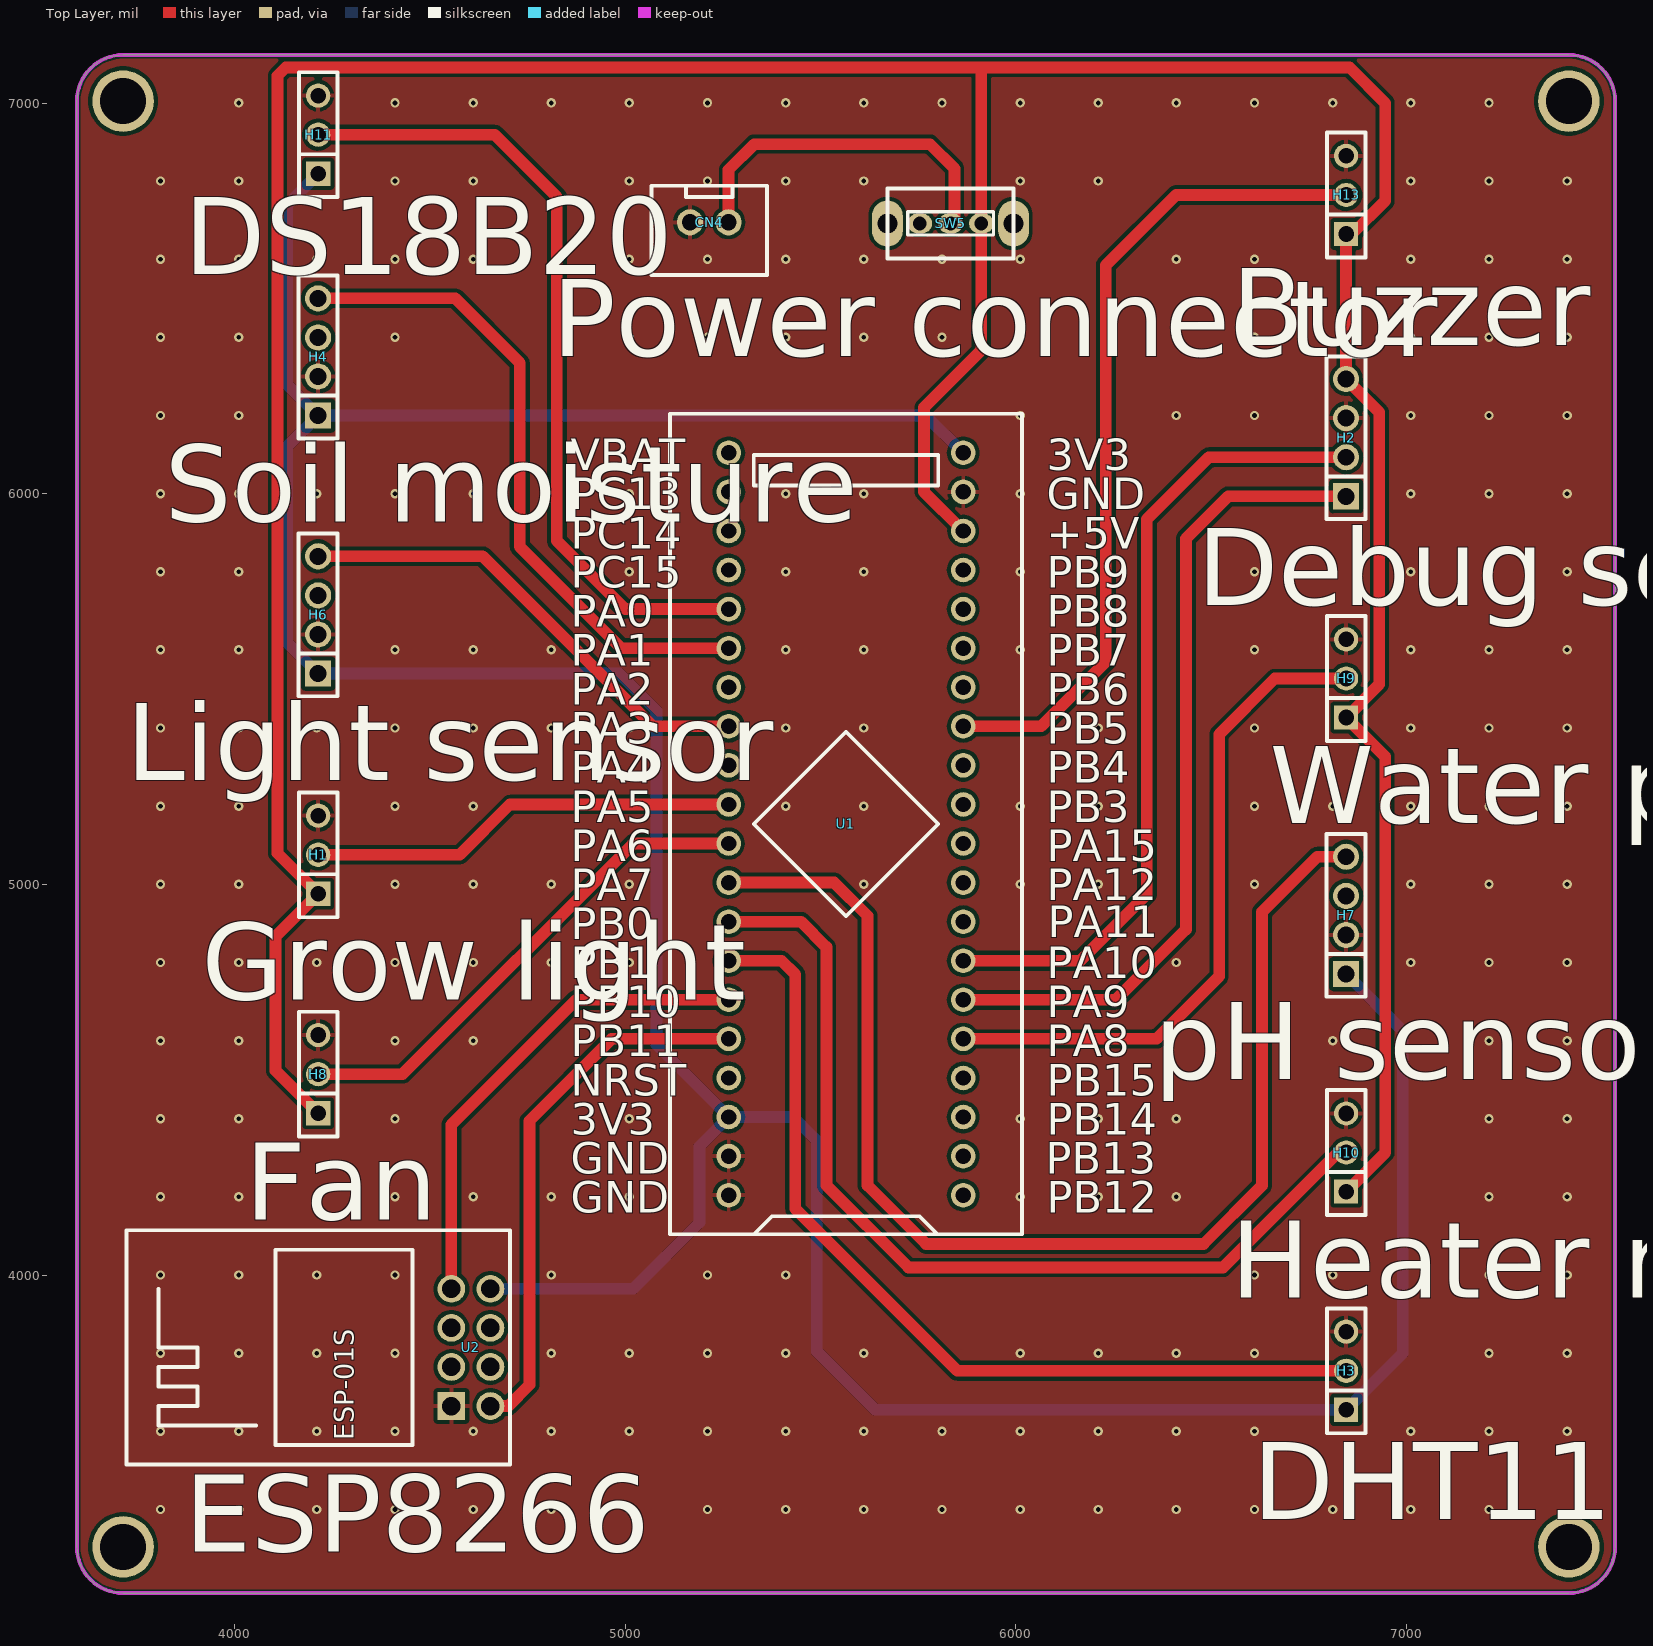
[diagram p0: Top Layer view]
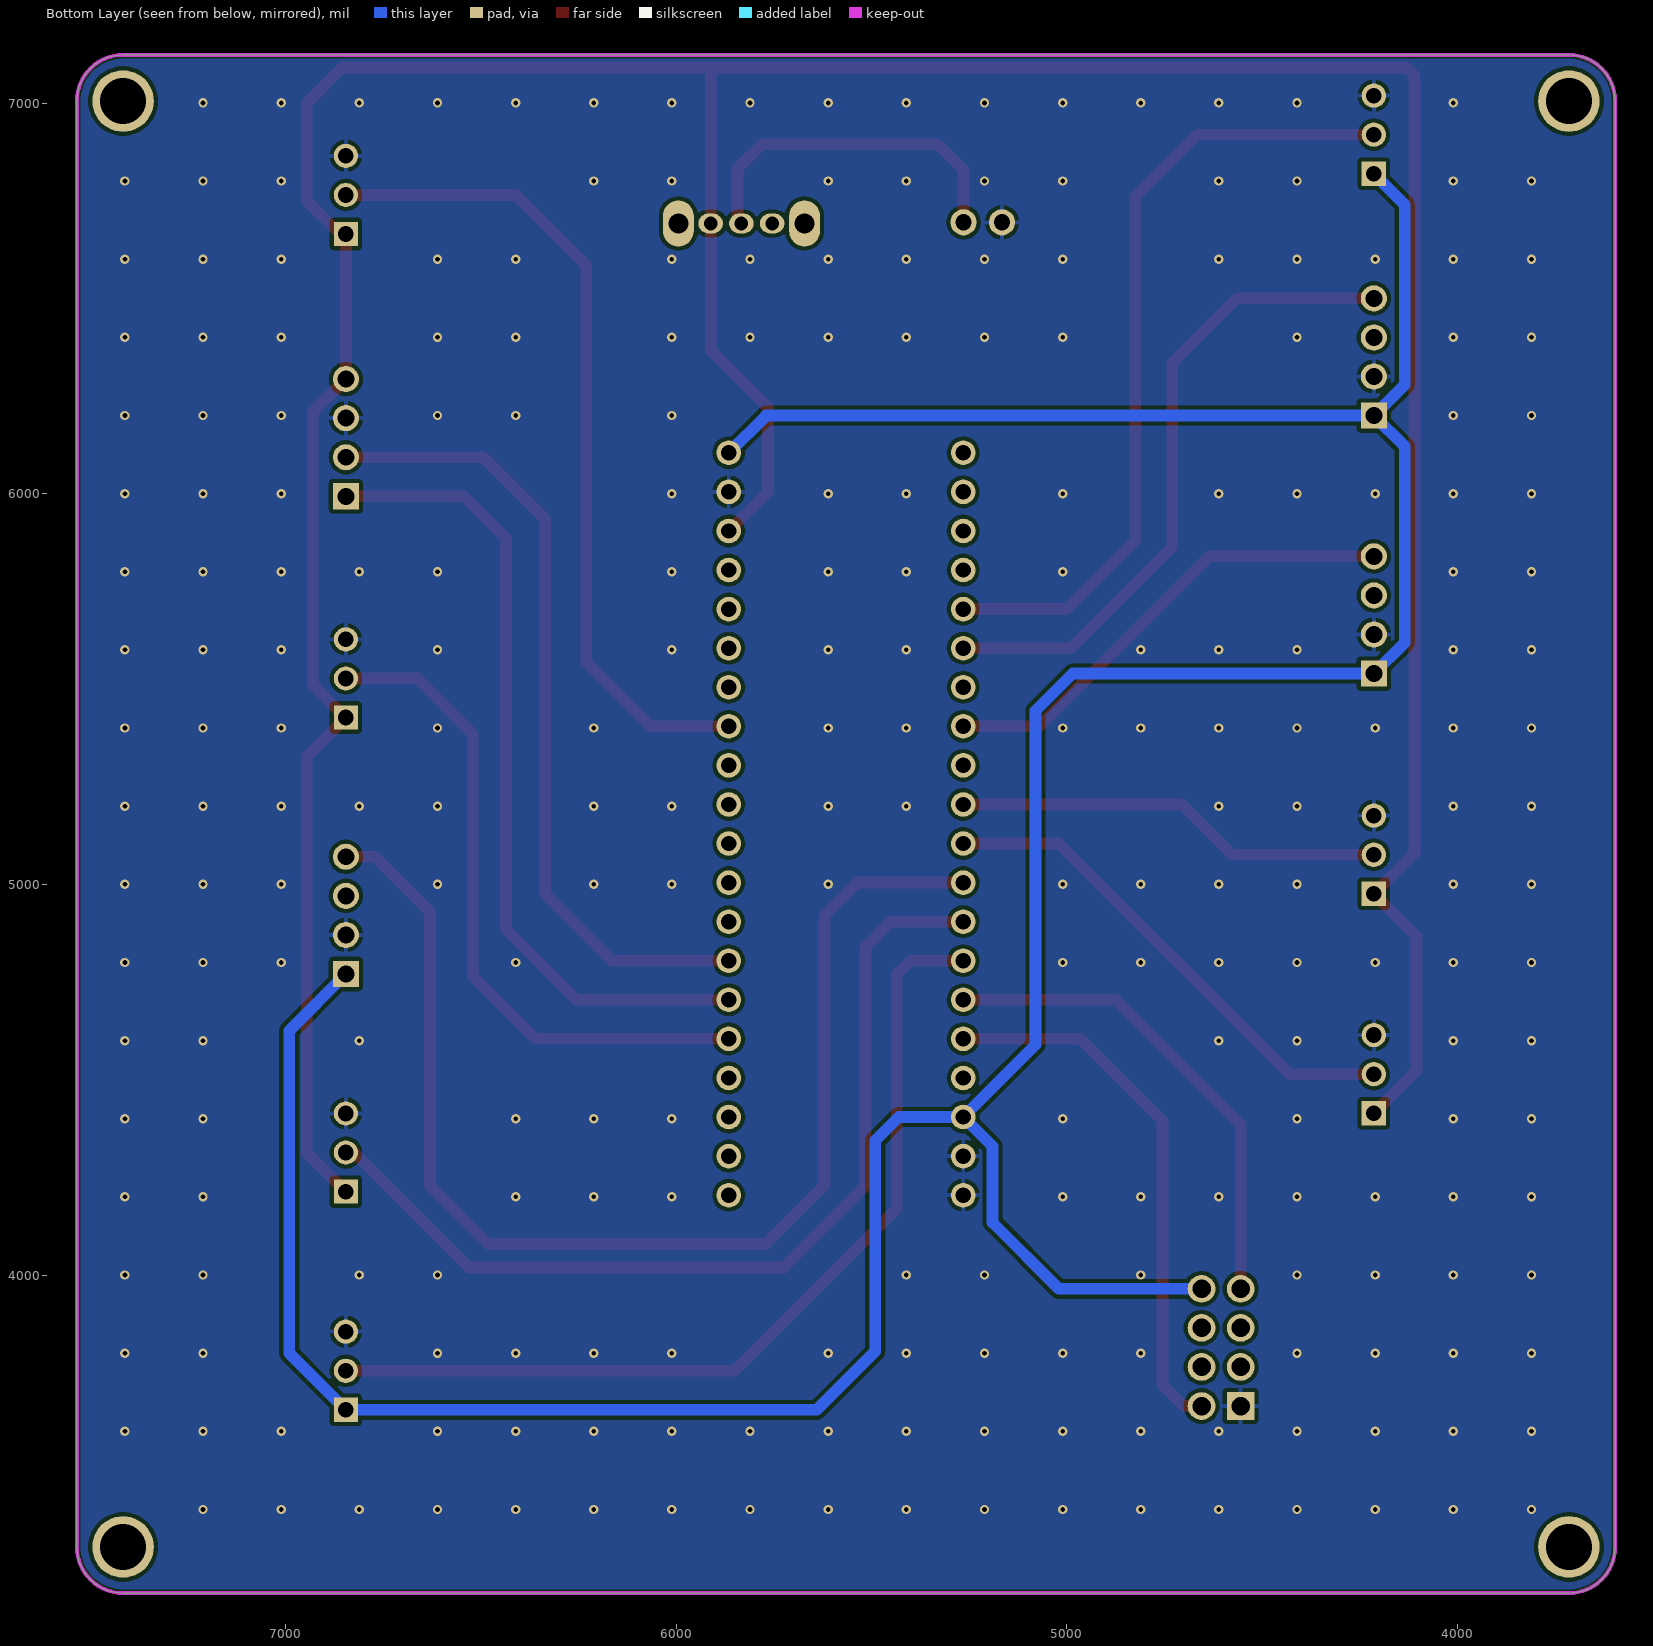
[diagram p1: Bottom Layer view, seen from below]
# Altium PCB MISC89003.pcbdoc
Units mil, origin at the board's own origin, x right, y up, seen from the top; angles counter-clockwise.
Board outline 3937.01 x 3937.01 mil, 2 copper layers (Top Layer, Bottom Layer), stack 62.206 mil thick; 15 components, 38 nets, 96 pads, 243 vias.

## Layer stack, top to bottom
Top Solder Mask Layer: solder mask 0.394, Dk 3.3
Top Layer: signal copper 1.379
Dielectric1: surface 59.449, FR4, Dk 4.5
Bottom Layer: signal copper 1.378
Bottom Solder Mask Layer: solder mask 0.394, Dk 3.3

## Board outline
3714.61,7123.5 ccw(c3714.61,7005.39) 3596.5,7005.39 3596.5,3304.61 ccw(c3714.61,3304.61) 3714.61,3186.5 7415.39,3186.5 ccw(c7415.39,3304.61) 7533.5,3304.61 7533.5,7005.39 ccw(c7415.39,7005.39) 7415.39,7123.5 3714.61,7123.5

## Design rules (kind name [scope] priority, off if disabled: settings)
BoardOutlineClearance copperThickness2oz_1 [All] p2 off: genericclearance=7.99 ignorepadtopadclearanceinfootprint=FALSE except(0: Arc-SplitContinuation Track-SplitContinuation SMDPad-SplitContinuation THPad-SplitContinuation Via-SplitContinuation Fill-SplitContinuation Region-SplitContinuation Poly-SplitContinuation Text-SplitContinuation Hole-SplitContinuation; 5.98: Arc-CutoutEdge Track-CutoutEdge SMDPad-CutoutEdge THPad-CutoutEdge Via-CutoutEdge Text-CutoutEdge; 6.9: Hole-OutlineEdge Hole-CutoutEdge; 10: Poly-OutlineEdge Poly-CutoutEdge; 11.81: Arc-OutlineEdge Track-OutlineEdge SMDPad-OutlineEdge THPad-OutlineEdge Via-OutlineEdge Fill-OutlineEdge Region-OutlineEdge Text-OutlineEdge Fill-CutoutEdge Region-CutoutEdge)
BoardOutlineClearance Plane_innerPlane_1 [All] p4 off: genericclearance=4.02 ignorepadtopadclearanceinfootprint=FALSE except(0: Arc-SplitContinuation Track-SplitContinuation SMDPad-SplitContinuation THPad-SplitContinuation Via-SplitContinuation Fill-SplitContinuation Region-SplitContinuation Poly-SplitContinuation Text-SplitContinuation Hole-SplitContinuation; 5.98: Arc-CutoutEdge Track-CutoutEdge SMDPad-CutoutEdge THPad-CutoutEdge Via-CutoutEdge Text-CutoutEdge; 6.9: Hole-OutlineEdge Hole-CutoutEdge; 10: Poly-OutlineEdge Poly-CutoutEdge; 11.81: Arc-OutlineEdge Track-OutlineEdge SMDPad-OutlineEdge THPad-OutlineEdge Via-OutlineEdge Fill-OutlineEdge Region-OutlineEdge Text-OutlineEdge Fill-CutoutEdge Region-CutoutEdge)
BoardOutlineClearance Copper_copperRegion_1 [All] p6 off: genericclearance=4.02 ignorepadtopadclearanceinfootprint=FALSE except(0: Arc-SplitContinuation Track-SplitContinuation SMDPad-SplitContinuation THPad-SplitContinuation Via-SplitContinuation Fill-SplitContinuation Region-SplitContinuation Poly-SplitContinuation Text-SplitContinuation Hole-SplitContinuation; 5.98: Arc-CutoutEdge Track-CutoutEdge SMDPad-CutoutEdge THPad-CutoutEdge Via-CutoutEdge Text-CutoutEdge; 6.9: Hole-OutlineEdge Hole-CutoutEdge; 10: Poly-OutlineEdge Poly-CutoutEdge; 11.81: Arc-OutlineEdge Track-OutlineEdge SMDPad-OutlineEdge THPad-OutlineEdge Via-OutlineEdge Fill-OutlineEdge Region-OutlineEdge Text-OutlineEdge Fill-CutoutEdge Region-CutoutEdge)
BoardOutlineClearance Copper_copperRegion_copperThickness1oz_1 [All] p8 off: genericclearance=4.02 ignorepadtopadclearanceinfootprint=FALSE except(0: Arc-SplitContinuation Track-SplitContinuation SMDPad-SplitContinuation THPad-SplitContinuation Via-SplitContinuation Fill-SplitContinuation Region-SplitContinuation Poly-SplitContinuation Text-SplitContinuation Hole-SplitContinuation; 5.98: Arc-CutoutEdge Track-CutoutEdge SMDPad-CutoutEdge THPad-CutoutEdge Via-CutoutEdge Text-CutoutEdge; 6.9: Hole-OutlineEdge Hole-CutoutEdge; 10: Poly-OutlineEdge Poly-CutoutEdge; 11.81: Arc-OutlineEdge Track-OutlineEdge SMDPad-OutlineEdge THPad-OutlineEdge Via-OutlineEdge Fill-OutlineEdge Region-OutlineEdge Text-OutlineEdge Fill-CutoutEdge Region-CutoutEdge)
BoardOutlineClearance Copper_copperRegion_Copper_copperRegion_1 [All] p10 off: genericclearance=4.02 ignorepadtopadclearanceinfootprint=FALSE except(0: Arc-SplitContinuation Track-SplitContinuation SMDPad-SplitContinuation THPad-SplitContinuation Via-SplitContinuation Fill-SplitContinuation Region-SplitContinuation Poly-SplitContinuation Text-SplitContinuation Hole-SplitContinuation; 5.98: Arc-CutoutEdge Track-CutoutEdge SMDPad-CutoutEdge THPad-CutoutEdge Via-CutoutEdge Text-CutoutEdge; 6.9: Hole-OutlineEdge Hole-CutoutEdge; 10: Poly-OutlineEdge Poly-CutoutEdge; 11.81: Arc-OutlineEdge Track-OutlineEdge SMDPad-OutlineEdge THPad-OutlineEdge Via-OutlineEdge Fill-OutlineEdge Region-OutlineEdge Text-OutlineEdge Fill-CutoutEdge Region-CutoutEdge)
BoardOutlineClearance copperThickness1oz_1 [All] p12: genericclearance=4.02 ignorepadtopadclearanceinfootprint=FALSE except(0: Arc-SplitContinuation Track-SplitContinuation SMDPad-SplitContinuation THPad-SplitContinuation Via-SplitContinuation Fill-SplitContinuation Region-SplitContinuation Poly-SplitContinuation Text-SplitContinuation Hole-SplitContinuation; 5.98: Arc-CutoutEdge Track-CutoutEdge SMDPad-CutoutEdge THPad-CutoutEdge Via-CutoutEdge Text-CutoutEdge; 6.9: Hole-OutlineEdge Hole-CutoutEdge; 10: Poly-OutlineEdge Poly-CutoutEdge; 11.81: Arc-OutlineEdge Track-OutlineEdge SMDPad-OutlineEdge THPad-OutlineEdge Via-OutlineEdge Fill-OutlineEdge Region-OutlineEdge Text-OutlineEdge Fill-CutoutEdge Region-CutoutEdge)
Clearance copperThickness2oz [All] p1 off: gap=7.99 ignorepadtopadclearanceinfootprint=FALSE except(5.98: SMDPad-Track SMDPad-SMDPad THPad-Track SMDPad-THPad THPad-THPad Track-Via SMDPad-Via THPad-Via Via-Via Fill-SMDPad Region-SMDPad Fill-THPad Region-THPad Fill-Via Region-Via Fill-Fill Fill-Region Region-Region Arc-Track Arc-SMDPad Arc-THPad Arc-Via Fill-Arc Region-Arc Arc-Arc Text-Track SMDPad-Text Text-THPad Text-Via Fill-Text Region-Text Arc-Text Text-Text; 6.9: Hole-Track Hole-SMDPad Hole-THPad Hole-Via Fill-Hole Region-Hole Hole-Arc Hole-Text; 10: Poly-Track Poly-SMDPad Poly-THPad Poly-Via Poly-Fill Poly-Region Poly-Poly Poly-Arc Poly-Text Poly-Hole; 11.81: Fill-Track Region-Track)
Clearance Plane_innerPlane [All] p3 off: gap=4.02 ignorepadtopadclearanceinfootprint=FALSE except(5.98: SMDPad-Track SMDPad-SMDPad THPad-Track SMDPad-THPad THPad-THPad Track-Via SMDPad-Via THPad-Via Via-Via Fill-SMDPad Region-SMDPad Fill-THPad Region-THPad Fill-Via Region-Via Fill-Fill Fill-Region Region-Region Arc-Track Arc-SMDPad Arc-THPad Arc-Via Fill-Arc Region-Arc Arc-Arc Text-Track SMDPad-Text Text-THPad Text-Via Fill-Text Region-Text Arc-Text Text-Text; 6.9: Hole-Track Hole-SMDPad Hole-THPad Hole-Via Fill-Hole Region-Hole Hole-Arc Hole-Text; 10: Poly-Track Poly-SMDPad Poly-THPad Poly-Via Poly-Fill Poly-Region Poly-Poly Poly-Arc Poly-Text Poly-Hole; 11.81: Fill-Track Region-Track)
Clearance Copper_copperRegion [All] p5 off: gap=4.02 ignorepadtopadclearanceinfootprint=FALSE except(5.98: SMDPad-Track SMDPad-SMDPad THPad-Track SMDPad-THPad THPad-THPad Track-Via SMDPad-Via THPad-Via Via-Via Fill-SMDPad Region-SMDPad Fill-THPad Region-THPad Fill-Via Region-Via Fill-Fill Fill-Region Region-Region Arc-Track Arc-SMDPad Arc-THPad Arc-Via Fill-Arc Region-Arc Arc-Arc Text-Track SMDPad-Text Text-THPad Text-Via Fill-Text Region-Text Arc-Text Text-Text; 6.9: Hole-Track Hole-SMDPad Hole-THPad Hole-Via Fill-Hole Region-Hole Hole-Arc Hole-Text; 10: Poly-Track Poly-SMDPad Poly-THPad Poly-Via Poly-Fill Poly-Region Poly-Poly Poly-Arc Poly-Text Poly-Hole; 11.81: Fill-Track Region-Track)
Clearance Copper_copperRegion_copperThickness1oz [All] p7 off: gap=4.02 ignorepadtopadclearanceinfootprint=FALSE except(5.98: SMDPad-Track SMDPad-SMDPad THPad-Track SMDPad-THPad THPad-THPad Track-Via SMDPad-Via THPad-Via Via-Via Fill-SMDPad Region-SMDPad Fill-THPad Region-THPad Fill-Via Region-Via Fill-Fill Fill-Region Region-Region Arc-Track Arc-SMDPad Arc-THPad Arc-Via Fill-Arc Region-Arc Arc-Arc Text-Track SMDPad-Text Text-THPad Text-Via Fill-Text Region-Text Arc-Text Text-Text; 6.9: Hole-Track Hole-SMDPad Hole-THPad Hole-Via Fill-Hole Region-Hole Hole-Arc Hole-Text; 10: Poly-Track Poly-SMDPad Poly-THPad Poly-Via Poly-Fill Poly-Region Poly-Poly Poly-Arc Poly-Text Poly-Hole; 11.81: Fill-Track Region-Track)
Clearance Copper_copperRegion_Copper_copperRegion [All] p9 off: gap=4.02 ignorepadtopadclearanceinfootprint=FALSE except(5.98: SMDPad-Track SMDPad-SMDPad THPad-Track SMDPad-THPad THPad-THPad Track-Via SMDPad-Via THPad-Via Via-Via Fill-SMDPad Region-SMDPad Fill-THPad Region-THPad Fill-Via Region-Via Fill-Fill Fill-Region Region-Region Arc-Track Arc-SMDPad Arc-THPad Arc-Via Fill-Arc Region-Arc Arc-Arc Text-Track SMDPad-Text Text-THPad Text-Via Fill-Text Region-Text Arc-Text Text-Text; 6.9: Hole-Track Hole-SMDPad Hole-THPad Hole-Via Fill-Hole Region-Hole Hole-Arc Hole-Text; 10: Poly-Track Poly-SMDPad Poly-THPad Poly-Via Poly-Fill Poly-Region Poly-Poly Poly-Arc Poly-Text Poly-Hole; 11.81: Fill-Track Region-Track)
Clearance copperThickness1oz [All] p11: gap=4.02 ignorepadtopadclearanceinfootprint=FALSE except(5.98: SMDPad-Track SMDPad-SMDPad THPad-Track SMDPad-THPad THPad-THPad Track-Via SMDPad-Via THPad-Via Via-Via Fill-SMDPad Region-SMDPad Fill-THPad Region-THPad Fill-Via Region-Via Fill-Fill Fill-Region Region-Region Arc-Track Arc-SMDPad Arc-THPad Arc-Via Fill-Arc Region-Arc Arc-Arc Text-Track SMDPad-Text Text-THPad Text-Via Fill-Text Region-Text Arc-Text Text-Text; 6.9: Hole-Track Hole-SMDPad Hole-THPad Hole-Via Fill-Hole Region-Hole Hole-Arc Hole-Text; 10: Poly-Track Poly-SMDPad Poly-THPad Poly-Via Poly-Fill Poly-Region Poly-Poly Poly-Arc Poly-Text Poly-Hole; 11.81: Fill-Track Region-Track)
DiffPairsRouting differentialPair [All] p1: maxlimit=6 minlimit=6 mostfreqgap=6 toplayer_minwidth=5 toplayer_prefwidth=10 toplayer_maxwidth=100 toplayer_mingap=6 toplayer_prefgap=6 toplayer_maxgap=6 bottomlayer_minwidth=5 bottomlayer_prefwidth=10 bottomlayer_maxwidth=100 bottomlayer_mingap=6 bottomlayer_prefgap=6 bottomlayer_maxgap=6 maxuncoupledlength=10
HoleToHoleClearance otherClearance [All] p1: gap=11.81 allowstackedmicrovias=TRUE
Length netLength [All] p1: minlimit=0 maxlimit=0
PasteMaskExpansion pasteMaskExpansion [All] p1: expansion=0
PlaneConnect innerPlane [All] p1: planeconnectstyle=Relief reliefexpansion=20 reliefentries=4 reliefconductorwidth=10 reliefairgap=10
PolygonConnect copperRegion_copperThickness1oz [All] p1 off: connectstyle=Relief reliefconductorwidth=10 reliefentries=4 polygonreliefangle="90 Angle" airgapwidth=10 via.connectstyle=Relief via.reliefconductorwidth=10 via.reliefentries=4 via.polygonreliefangle="90 Angle" via.airgapwidth=10
PolygonConnect copperRegion_Copper_copperRegion [All] p2 off: connectstyle=Relief reliefconductorwidth=10 reliefentries=4 polygonreliefangle="90 Angle" airgapwidth=10 via.connectstyle=Relief via.reliefconductorwidth=10 via.reliefentries=4 via.polygonreliefangle="90 Angle" via.airgapwidth=10
PolygonConnect copperRegion [All] p3: connectstyle=Relief reliefconductorwidth=10 reliefentries=4 polygonreliefangle="90 Angle" airgapwidth=10 via.connectstyle=Relief via.reliefconductorwidth=10 via.reliefentries=4 via.polygonreliefangle="90 Angle" via.airgapwidth=10
RoutingVias viaSize [All] p1: holewidth=12.01 width=24.02 viastyle="Through Hole" minholewidth=11.81 minwidth=19.68 maxholewidth=248.03 maxwidth=393.7
SolderMaskExpansion solderMaskExpansion [IsVia] p1: expansion=-1000 istentingtop=TRUE
SolderMaskExpansion solderMaskExpansion [All] p2: expansion=2 istentingtop=FALSE
Width copperThickness2oz_2 [All] p1 off: maxlimit=100 minlimit=8 preferedwidth=10
Width copperThickness1oz_2 [All] p2: maxlimit=100 minlimit=5 preferedwidth=10

## Components (designator, comment, footprint, x,y, rotation, side; value= is the part's Value field where it differs from the comment)
CN4 "XH2.54*2P_straight" CONN-TH_2P-P2.50-XH2.54-2P 5215,6695 r0 top
H1 "" HDR-TH_3P-P2.54-V-F 4214,5076.28 r90 top
H2 "" HDR-TH_4P-P2.54-V-F 6845,6143.71 r90 top
H3 "" HDR-TH_3P-P2.54-V-F 6845,3755.57 r90 top
H4 "" HDR-TH_4P-P2.54-V-F 4214,6350.33 r90 top
H6 "" HDR-TH_4P-P2.54-V-F 4214,5690.14 r90 top
H7 "" HDR-TH_4P-P2.54-V-F 6845,4921.1 r90 top
H8 "" HDR-TH_3P-P2.54-V-F 4214,4514.73 r90 top
H9 "" HDR-TH_3P-P2.54-V-F 6845,5527.48 r90 top
H10 "" HDR-TH_3P-P2.54-V-F 6845,4314.12 r90 top
H11 "" HDR-TH_3P-P2.54-V-F 4214,6919.25 r90 top
H13 "" HDR-TH_3P-P2.54-V-F 6845,6765 r90 top
SW5 "" 拨动开关 5837.9,6692.05 r180 top
U1 "STM32F103C8T6-Card" CONN-TH_L53.3-W22.9_STM32F103C8T6-CARD 5565,5155 r90 top
U2 "ESP-01S" WIFIM-TH_ESP-01S 4605,3815.3 r90 top

## Footprints (in the part's own frame and the unit in brackets; to place one, negate y for a bottom-side part, rotate by r counter-clockwise, add the part's x,y. Pads: shape width x height; smd on the part's side, far side on the other; paste and mask are expansions set on the pad)
CONN-TH_2P-P2.50-XH2.54-2P [mm]
  round 1.7 hole 1.05 paste+0 mask+0.05: 1(1.25,0) 2(-1.25,0)
  silkscreen extent -3.75,-3.42 3.75,2.37
CONN-TH_L53.3-W22.9_STM32F103C8T6-CARD [mm]
  round 1.6 hole 1: 1(-24.13,-7.62) 2(-21.59,-7.62) 3(-19.05,-7.62) 4(-16.51,-7.62) 5(-13.97,-7.62) 6(-11.43,-7.62) 7(-8.89,-7.62) 8(-6.35,-7.62) 9(-3.81,-7.62) 10(-1.27,-7.62) 11(1.27,-7.62) 12(3.81,-7.62) 13(6.35,-7.62) 14(8.89,-7.62) 15(11.43,-7.62) 16(13.97,-7.62) 17(16.51,-7.62) 18(19.05,-7.62) 19(21.59,-7.62) 20(24.13,-7.62) 21(24.13,7.62) 22(21.59,7.62) 23(19.05,7.62) 24(16.51,7.62) 25(13.97,7.62) 26(11.43,7.62) 27(8.89,7.62) 28(6.35,7.62) 29(3.81,7.62) 30(1.27,7.62) 31(-1.27,7.62) 32(-3.81,7.62) 33(-6.35,7.62) 34(-8.89,7.62) 35(-11.43,7.62) 36(-13.97,7.62) 37(-16.51,7.62) 38(-19.05,7.62) 39(-21.59,7.62) 40(-24.13,7.62)
  silkscreen extent -26.67,-11.43 26.67,11.43
HDR-TH_3P-P2.54-V-F [mil]
  rect 62x62 hole 40.16: 1(-100,0)
  round 62 hole 40.16: 2(0,0) 3(100,0)
  silkscreen extent -160,-49 160,49
HDR-TH_4P-P2.54-V-F [mm]
  rect 1.7x1.7 hole 1.1: 1(-3.81,0)
  round 1.7 hole 1.1: 2(-1.27,0) 3(1.27,0) 4(3.81,0)
  silkscreen extent -5.29,-1.27 5.29,1.27
WIFIM-TH_ESP-01S [mm]
  rect 1.8x1.8 hole 1.2: 1(-3.81,1.27)
  round 1.8 hole 1.2: 2(-1.27,1.27) 3(1.27,1.27) 4(3.81,1.27) 5(3.81,-1.27) 6(1.27,-1.27) 7(-1.27,-1.27) 8(-3.81,-1.27)
  silkscreen extent -7.62,-2.54 7.62,22.4
拨动开关 [mil]
  oval 63x51.2 hole 35.4 paste+0 mask+2: 1(-73.4,0) 2(5,0) 3(84,0)
  oval 78.7x118.1 hole 51.2 paste+0 mask+2: 4(166.7,0) 5(-156.1,0)
  silkscreen extent -156,-90 167,90

## Free pads (board coordinates)
  round 157.48 hole 118.11: 1(3714.61,7005.39) 1(3714.61,3304.61) 1(7415.39,7005.39) 1(7415.39,3304.61)

## Via types
v1: diameter 24.02, hole 12, Top Layer to Bottom Layer, 243 vias

## Nets (pads, with @x,y where several pads share a name; then routed paths per layer and width w, separated by ;. In a path a pad name is that pad's centre, name@x,y a point inside that pad or via, vN(x,y) a via of type N, cw(c..) or ccw(c..) an arc to the next point about the centre after c; other vN are vias at no path point)
$1N17118: CN4.1 SW5.2 | length 906.3
  Top Layer w30: CN4.1 5264.22,6829.22 5330,6895 5780,6895 5842.9,6832.1 SW5.2@5842.9,6692.05
+5V: H1.1 H2.4 H8.1 H9.1 H10.1 H13.1 SW5.1 U1.18 | length 9949
  Top Layer w30: H8.1 4105,4523.73 4105,4867.28 H1.1 4110,5080.28 4110,7070 4131.21,7091.21 5909.46,7091.21 ; U1.18 5764.5,6005.5 5764.5,6220.75 5911.3,6367.55 SW5.1 5911.3,7089.37 5909.46,7091.21 ; H10.1 6945,4314.12 6945,5327.48 H9.1 6930,5512.48 6930,6208.71 H2.4 H13.1 6860,6665 6945,6750 6945,7000 6853.79,7091.21 5909.46,7091.21
GND: CN4.2 H1.3 H2.3 H3.3 H4.2 H6.2 H7.2 H8.3 H9.3 H10.3 H11.3 H13.3 U1.19 U1.39 U1.40 U2.1
  other v1: 3810.6,3400.6 4010.6,3400.6 4210.6,3400.6 4410.6,3400.6 4610.6,3400.6 4810.6,3400.6 5010.6,3400.6 5210.6,3400.6 5410.6,3400.6 5610.6,3400.6 5810.6,3400.6 6010.6,3400.6 6210.6,3400.6 6410.6,3400.6 6610.6,3400.6 6810.6,3400.6 7010.6,3400.6 7210.6,3400.6 3810.6,3600.6 4010.6,3600.6 4210.6,3600.6 4410.6,3600.6 4610.6,3600.6 4810.6,3600.6 5010.6,3600.6 5210.6,3600.6 5410.6,3600.6 5610.6,3600.6 5810.6,3600.6 6010.6,3600.6 6210.6,3600.6 6410.6,3600.6 6610.6,3600.6 7010.6,3600.6 7210.6,3600.6 7410.6,3600.6 3810.6,3800.6 4010.6,3800.6 4210.6,3800.6 4410.6,3800.6 4810.6,3800.6 5010.6,3800.6 5210.6,3800.6 5410.6,3800.6 5610.6,3800.6 6010.6,3800.6 6210.6,3800.6 6410.6,3800.6 6610.6,3800.6 7210.6,3800.6 7410.6,3800.6 3810.6,4000.6 4010.6,4000.6 4210.6,4000.6 4410.6,4000.6 4810.6,4000.6 5210.6,4000.6 5410.6,4000.6 6610.6,4000.6 6810.6,4000.6 7210.6,4000.6 7410.6,4000.6 3810.6,4200.6 4010.6,4200.6 4210.6,4200.6 4410.6,4200.6 4610.6,4200.6 4810.6,4200.6 5010.6,4200.6 6010.6,4200.6 6210.6,4200.6 6410.6,4200.6 7210.6,4200.6 7410.6,4200.6 3810.6,4400.6 4010.6,4400.6 4410.6,4400.6 5010.6,4400.6 6010.6,4400.6 6210.6,4400.6 6410.6,4400.6 7210.6,4400.6 7410.6,4400.6 3810.6,4600.6 4010.6,4600.6 4410.6,4600.6 4610.6,4600.6 6810.6,4600.6 7210.6,4600.6 7410.6,4600.6 3810.6,4800.6 4010.6,4800.6 4210.6,4800.6 4410.6,4800.6 4610.6,4800.6 4810.6,4800.6 5010.6,4800.6 6410.6,4800.6 7010.6,4800.6 7210.6,4800.6 7410.6,4800.6 3810.6,5000.6 4010.6,5000.6 4410.6,5000.6 4610.6,5000.6 4810.6,5000.6 5010.6,5000.6 5610.6,5000.6 6010.6,5000.6 6210.6,5000.6 6610.6,5000.6 7010.6,5000.6 7210.6,5000.6 7410.6,5000.6 3810.6,5200.6 4010.6,5200.6 4410.6,5200.6 4610.6,5200.6 5410.6,5200.6 5610.6,5200.6 6010.6,5200.6 6210.6,5200.6 6610.6,5200.6 6810.6,5200.6 7010.6,5200.6 7210.6,5200.6 7410.6,5200.6 3810.6,5400.6 4010.6,5400.6 4210.6,5400.6 4410.6,5400.6 4610.6,5400.6 4810.6,5400.6 5010.6,5400.6 5410.6,5400.6 5610.6,5400.6 6210.6,5400.6 6610.6,5400.6 7010.6,5400.6 7210.6,5400.6 7410.6,5400.6 3810.6,5600.6 4010.6,5600.6 4410.6,5600.6 4610.6,5600.6 4810.6,5600.6 5410.6,5600.6 5610.6,5600.6 6010.6,5600.6 6610.6,5600.6 7010.6,5600.6 7210.6,5600.6 7410.6,5600.6 3810.6,5800.6 4010.6,5800.6 5010.6,5800.6 5410.6,5800.6 5610.6,5800.6 6010.6,5800.6 6610.6,5800.6 6810.6,5800.6 7010.6,5800.6 7210.6,5800.6 7410.6,5800.6 3810.6,6000.6 4010.6,6000.6 4210.6,6000.6 4410.6,6000.6 4610.6,6000.6 5010.6,6000.6 5410.6,6000.6 5610.6,6000.6 6010.6,6000.6 7010.6,6000.6 7210.6,6000.6 7410.6,6000.6 3810.6,6200.6 4010.6,6200.6 6010.6,6200.6 6410.6,6200.6 6610.6,6200.6 7010.6,6200.6 7210.6,6200.6 7410.6,6200.6 3810.6,6400.6 4010.6,6400.6 4410.6,6400.6 5010.6,6400.6 5210.6,6400.6 5410.6,6400.6 5610.6,6400.6 5810.6,6400.6 6010.6,6400.6 6410.6,6400.6 6610.6,6400.6 7010.6,6400.6 7210.6,6400.6 7410.6,6400.6 3810.6,6600.6 4010.6,6600.6 4210.6,6600.6 4410.6,6600.6 4610.6,6600.6 5010.6,6600.6 5210.6,6600.6 5410.6,6600.6 5610.6,6600.6 5810.6,6600.6 6010.6,6600.6 6410.6,6600.6 6610.6,6600.6 7010.6,6600.6 7210.6,6600.6 7410.6,6600.6 3810.6,6800.6 4010.6,6800.6 4410.6,6800.6 4610.6,6800.6 5010.6,6800.6 5210.6,6800.6 5410.6,6800.6 5610.6,6800.6 6010.6,6800.6 6210.6,6800.6 7010.6,6800.6 7210.6,6800.6 7410.6,6800.6 4010.6,7000.6 4410.6,7000.6 4610.6,7000.6 4810.6,7000.6 5010.6,7000.6 5210.6,7000.6 5410.6,7000.6 5610.6,7000.6 5810.6,7000.6 6010.6,7000.6 6210.6,7000.6 6410.6,7000.6 6610.6,7000.6 6810.6,7000.6 7010.6,7000.6 7210.6,7000.6
NRST: U1.37
PA0: H11.2 U1.25 | length 2069.4
  Top Layer w30: H11.2 4665.75,6919.25 4825,6760 4825,5880 5000,5705 U1.25
PA1: H4.4 U1.26 | length 1697.2
  Top Layer w30: H4.4 4564.67,6500.33 4730,6335 4730,5865 4990,5605 U1.26
PA2: U1.27
PA3: H6.4 U1.28 | length 1231.2
  Top Layer w30: H6.4 4634.86,5840.14 5070,5405 U1.28
PA4: U1.29
PA5: H1.2 U1.30 | length 1104.3
  Top Layer w30: H1.2 4576.28,5076.28 4705,5205 U1.30
PA6: H8.2 U1.31 | length 1295.5
  Top Layer w30: H8.2 4429.73,4514.73 5020,5105 U1.31
PA7: H7.4 U1.32 | length 3187.9
  Top Layer w30: U1.32 5535,5005 5620,4920 5620,4230 5770,4080 6480,4080 6630,4230 6630,4930 6771.1,5071.1 H7.4
PA8: H9.2 U1.5 | length 1725.3
  Top Layer w30: U1.5 6360,4605 6520,4765 6520,5385 6662.48,5527.48 H9.2
PA9: H2.1 U1.6 | length 2099.6
  Top Layer w30: U1.6 6255,4705 6435,4885 6435,5885 6543.71,5993.71 H2.1
PA10: H2.2 U1.7 | length 2076.2
  Top Layer w30: U1.7 6165,4805 6335,4975 6335,5935 6493.71,6093.71 H2.2
PA11: U1.8
PA12: U1.9
PA15: U1.10
PB0: H10.2 U1.33 | length 2425.7
  Top Layer w30: U1.33 5450,4905 5515,4840 5515,4230 5725,4020 6530,4020 6824.12,4314.12 H10.2
PB1: H3.2 U1.34 | length 2366.2
  Top Layer w30: U1.34 5400,4805 5435,4770 5435,4170 5849.43,3755.57 H3.2
PB3: U1.11
PB4: U1.12
PB5: H13.2 U1.13 | length 2137.9
  Top Layer w30: U1.13 6065,5405 6230,5570 6230,6585 6410,6765 H13.2
PB6: U1.14
PB7: U1.15
PB8: U1.16
PB9: U1.17
PB10: U1.35 U2.4 | length 1262.2
  Top Layer w30: U2.4 4555,4385 4875,4705 U1.35
PB11: U1.36 U2.8 | length 1394.6
  Top Layer w30: U2.8 4700.3,3665.3 4755,3720 4755,4395 4965,4605 U1.36
PB12: U1.1
PB13: U1.2
PB14: U1.3
PB15: U1.4
PC13: U1.22
PC14: U1.23
PC15: U1.24
VBAT: U1.21
VCC: H3.1 H4.1 H6.1 H7.1 H11.1 U1.20 U1.38 U2.5 | length 9471.3
  Bottom Layer w30: H11.1 4135,6740.25 4135,6279.33 H4.1 ; U2.5 5020.3,3965.3 5190,4135 5190,4330 U1.38 ; U1.20 5769.67,6200.33 H4.1 ; H7.1 6990,4626.1 6990,3800.57 H3.1 5639.43,3655.57 5490,3805 5490,4345 5430,4405 U1.38 ; H4.1 4135,6121.33 4135,5619.14 H6.1 4984.86,5540.14 5080,5445 5080,4590 U1.38
pads on no net: H4.3 H6.3 H7.3 SW5.3 SW5.4 SW5.5 U2.2 U2.3 U2.6 U2.7

## Polygon pours and split planes (outlines as drawn)
GND on Bottom Layer (solid, remove dead copper, pour order 4): 3525,7245 3525,3080 7700,3080 7700,7245
GND on Top Layer (solid, remove dead copper, pour order 2): 3000,7415 3000,3000 7930,3000 7930,7415
GND on Top Layer (solid, remove dead copper, pour order 4): 3285,7285 3285,3165 7970,3165 7970,7285
GND on Bottom Layer (solid, remove dead copper, pour order 6): 3425,7280 3425,3115 7830,3115 7830,7280

## Keep-outs
Board Outline Layer:
  the board outline again, w10

## Silkscreen, mask and mechanical layers (free items; w line width, h text height)
Top Silkscreen Layer:
  text "DS18B20" at 3871.9,6562.37 h196.85
  text "Buzzer" at 6551.81,6380.14 h196.85
  text "Power connector" at 4812.87,6351.57 h196.85
  text "VBAT" at 4860.95,6060 h80
  text "3V3" at 6079.16,6060 h80
  text "PC13" at 4860.95,5960 h80
  text "GND" at 6079.16,5960 h80
  text "Soil moisture" at 3820.75,5928.67 h196.85
  text "PC14" at 4860.95,5860 h80
  text "+5V" at 6079.16,5860 h80
  text "PC15" at 4860.95,5760 h80
  text "PB9" at 6079.16,5760 h80
  text "Debug serial port" at 6464.27,5714.89 h196.85
  text "PA0" at 4860.95,5660 h80
  text "PB8" at 6079.16,5660 h80
  text "PA1" at 4860.95,5560 h80
  text "PB7" at 6079.16,5560 h80
  text "PA2" at 4860.95,5460 h80
  text "PB6" at 6079.16,5460 h80
  text "PA3" at 4860.95,5360 h80
  text "PB5" at 6079.16,5360 h80
  text "Light sensor" at 3723.07,5266.39 h196.85
  text "PA4" at 4860.95,5260 h80
  text "PB4" at 6079.16,5260 h80
  text "PA5" at 4860.95,5160 h80
  text "PB3" at 6079.16,5160 h80
  text "Water pump" at 6649.34,5156.94 h196.85
  text "PA6" at 4860.95,5060 h80
  text "PA15" at 6079.16,5060 h80
  text "PA7" at 4860.95,4960 h80
  text "PA12" at 6079.16,4960 h80
  text "PA11" at 6080.95,4865 h80
  text "PB0" at 4860.95,4860 h80
  text "PB1" at 4860.95,4760 h80
  text "PA10" at 6079.16,4760 h80
  text "Grow light" at 3916.34,4704.83 h196.85
  text "PB10" at 4860.95,4660 h80
  text "PA9" at 6079.16,4660 h80
  text "PB11" at 4860.95,4560 h80
  text "PA8" at 6079.16,4560 h80
  text "pH sensor" at 6354.22,4501.53 h196.85
  text "NRST" at 4860.95,4460 h80
  text "PB15" at 6079.16,4460 h80
  text "3V3" at 4860.95,4360 h80
  text "PB14" at 6079.16,4360 h80
  text "GND" at 4860.95,4260 h80
  text "PB13" at 6075.95,4260 h80
  text "GND" at 4860.95,4160 h80
  text "PB12" at 6079.16,4160 h80
  text "Fan" at 4026.99,4142.09 h196.85
  text "Heater rod" at 6549.54,3942.98 h196.85
  text "DHT11" at 6606.39,3375.18 h196.85
  text "ESP8266" at 3872.2,3292.86 h196.85